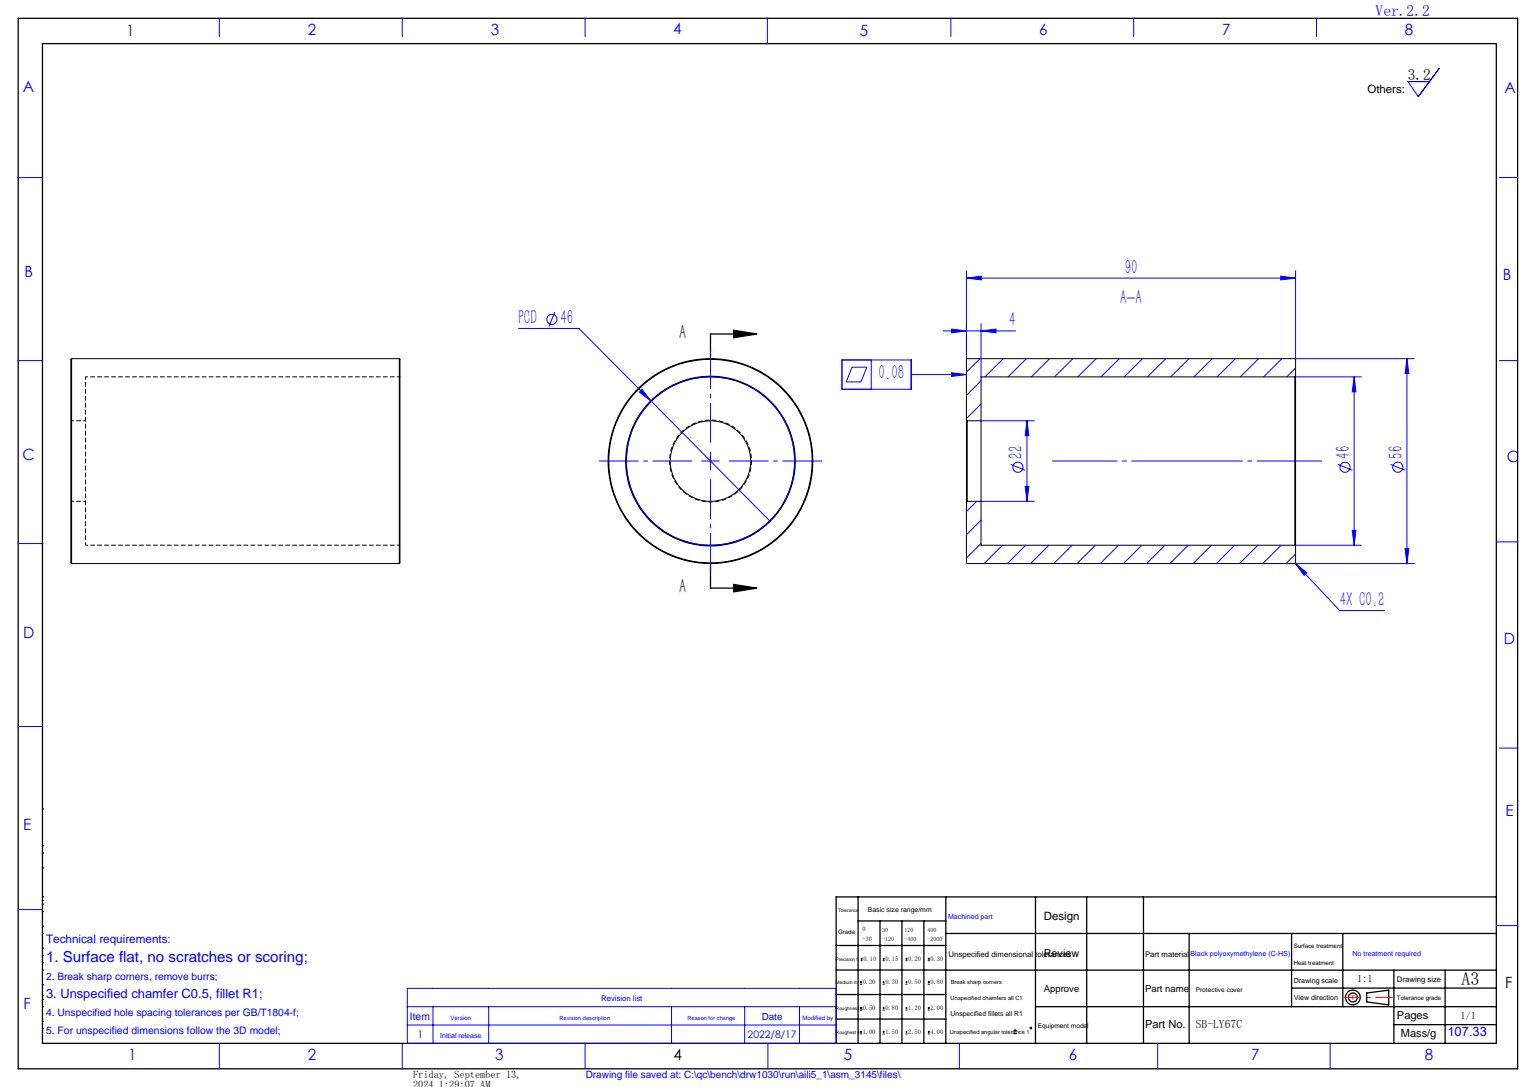
SolidWorks part; units mm, degrees
material "黑色赛钢(C-HS)"
ref_plane "前视基准面" through (0, 0, 0) normal (0, 0, 1) x (1, 0, 0)
ref_plane "上视基准面" through (0, 0, 0) normal (0, 1, 0) x (1, 0, 0)
ref_plane "右视基准面" through (0, 0, 0) normal (1, 0, 0) x (0, 0, -1)
sketch "草图2" plane through (0, 0, 0) normal (0, 0, 1) x (1, 0, 0)
  circle A0 centre (0, 0) radius 36.7857
sketch "草图3" plane through (0, 0, 0) normal (0, 1, 0) x (1, 0, 0)
  circle A0 centre (0, 0) radius 23
  circle A1 centre (0, 0) radius 28
  dimension "D1" = 46
  dimension "D2" = 56
extrude "凸台-拉伸1" add sketch "草图3" along normal blind 90
sketch "草图4" plane through (0, 90, 0) normal (0, -1, 0) x (1, 0, 0)
  circle A0 centre (0, 0) radius 23.5
  circle A1 centre (0, 0) radius 11
  dimension "D1" = 22
  dimension "D2" = 47
extrude "凸台-拉伸2" add sketch "草图4" along normal blind 4
chamfer "倒角1" distance 0.2 angle 45 4 edges at (0, 90, -11) (0, 0, 23) (0, 90, 28) (0, 0, 28)
